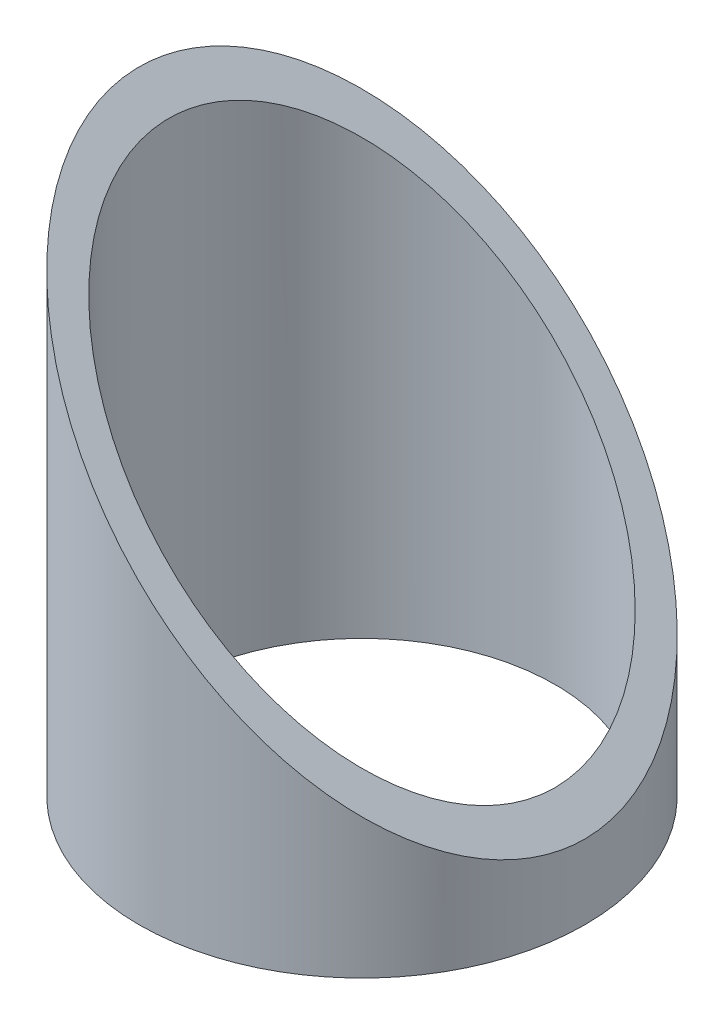
SolidWorks part; units mm, degrees
material "Q235"
ref_plane "Front Plane" through (0, 0, 0) normal (0, 0, 1) x (1, 0, 0)
ref_plane "Top Plane" through (0, 0, 0) normal (0, 1, 0) x (1, 0, 0)
ref_plane "Right Plane" through (0, 0, 0) normal (1, 0, 0) x (0, 0, -1)
sketch "Sketch1" plane through (0, 0, 0) normal (0, 1, 0) x (1, 0, 0)
  circle A0 centre (0, 0) radius 30
  circle A1 centre (0, 0) radius 26
  dimension "D1" = 4
  dimension "D2" = 60
extrude "Boss-Extrude1" add sketch "Sketch1" along normal blind 70
sketch "Sketch2" plane through (0, 0, 0) normal (0, 0, 1) x (1, 0, 0)
  line L0 (-30, 70) -> (33.2123, 6.7877)
  line L1 (30, 70) -> (-30, 70) construction
  dimension "D1" = 45
extrude "Cut-Extrude1" cut sketch "Sketch2" against normal through all both and the other way through all
